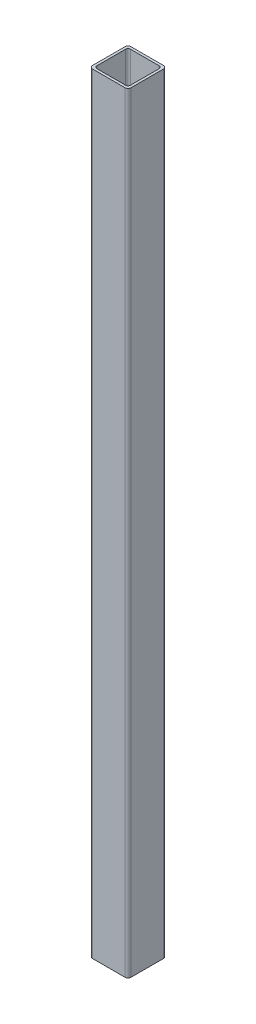
from build123d import *

# Parameters (mm, degrees)
BOSS_EXTRUDE1_DEPTH = 1000


with BuildPart() as part:
    # Sketch2 → Boss-Extrude1 (new, symmetric)
    with BuildSketch(Plane(origin=(0, 0, 0), x_dir=(1, 0, 0), z_dir=(0, 1, 0))):
        with BuildLine():
            Line((7.875, -1.525), (92.125, -1.525))
            ThreePointArc((92.125, -1.525), (97.693465902, 0.781534098), (100, 6.35))
            Line((100, 6.35), (100, 90.6))
            ThreePointArc((100, 90.6), (97.693465902, 96.168465902), (92.125, 98.475))
            Line((92.125, 98.475), (7.875, 98.475))
            ThreePointArc((7.875, 98.475), (2.306534098, 96.168465902), (0, 90.6))
            Line((0, 90.6), (0, 6.35))
            ThreePointArc((0, 6.35), (2.306534098, 0.781534098), (7.875, -1.525))
        make_face()
        with BuildLine():
            Line((12.6, 4.775), (87.4, 4.775))
            ThreePointArc((87.4, 4.775), (91.854772721, 6.620227279), (93.7, 11.075))
            Line((93.7, 11.075), (93.7, 85.875))
            ThreePointArc((93.7, 85.875), (91.854772721, 90.329772721), (87.4, 92.175))
            Line((87.4, 92.175), (12.6, 92.175))
            ThreePointArc((12.6, 92.175), (8.145227279, 90.329772721), (6.3, 85.875))
            Line((6.3, 85.875), (6.3, 11.075))
            ThreePointArc((6.3, 11.075), (8.145227279, 6.620227279), (12.6, 4.775))
        make_face(mode=Mode.SUBTRACT)
    extrude(amount=BOSS_EXTRUDE1_DEPTH, both=True)


solid = part.part
